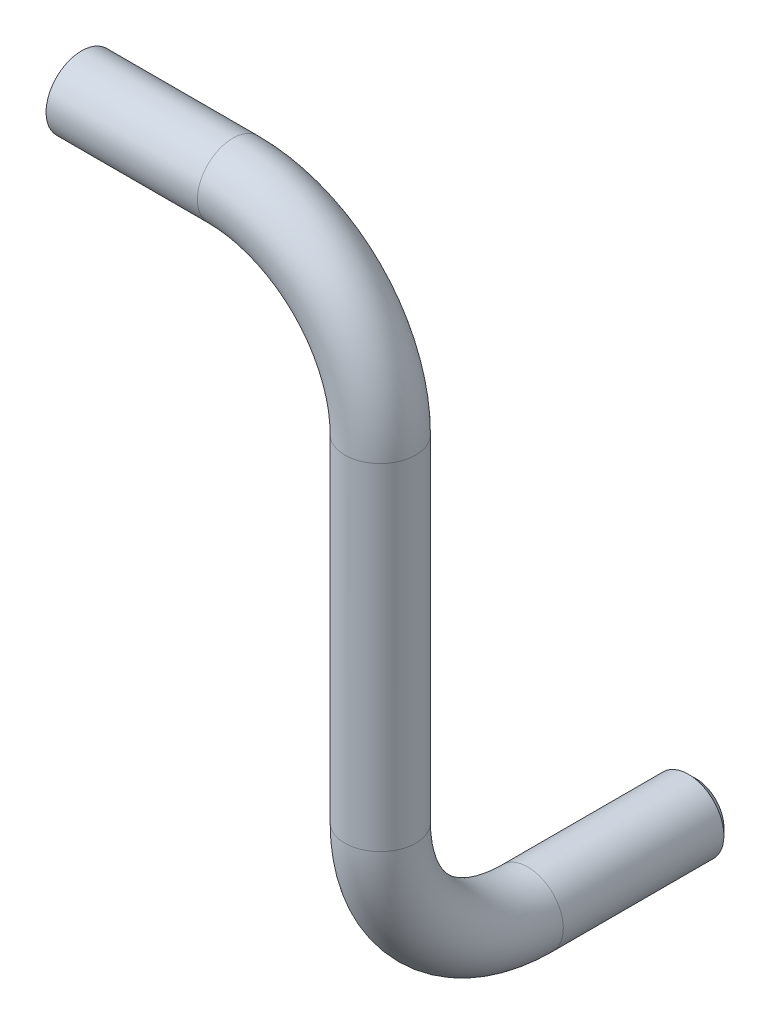
from build123d import *

# Parameters (mm, degrees)
SWEEP1_PROFILE_R = 9.5
CHAMFER1_SIZE    = 2


with BuildPart() as part:
    # Sweep1: sweep along a curve in space
    with BuildLine() as sweep1_path:
        Line((0, 0, 0), (40.5, 0, 0))
        ThreePointArc((40.5, 0, 0), (68.430717857, -11.569282143, 0), (80, -39.5, 0))
        Line((80, -39.5, 0), (80, -129.5, 0))
        ThreePointArc((80, -129.5, 0), (80, -157.430717857, -11.569282143), (80, -169, -39.5))
        Line((80, -169, -39.5), (80, -169, -84.5))
    # Sweep1 profile (on start of the path) → Sweep1 (sweep)
    with BuildSketch(Plane(origin=(0, 0, 0), x_dir=(0, 0, 1), z_dir=(1, 0, 0))):
        Circle(SWEEP1_PROFILE_R)
    sweep(path=sweep1_path.line)

    # Chamfer1
    chamfer1_edges = [part.edges().sort_by_distance(p)[0] for p in [
        (80, -159.5, -84.5),
    ]]
    chamfer(chamfer1_edges, length=CHAMFER1_SIZE)


solid = part.part
